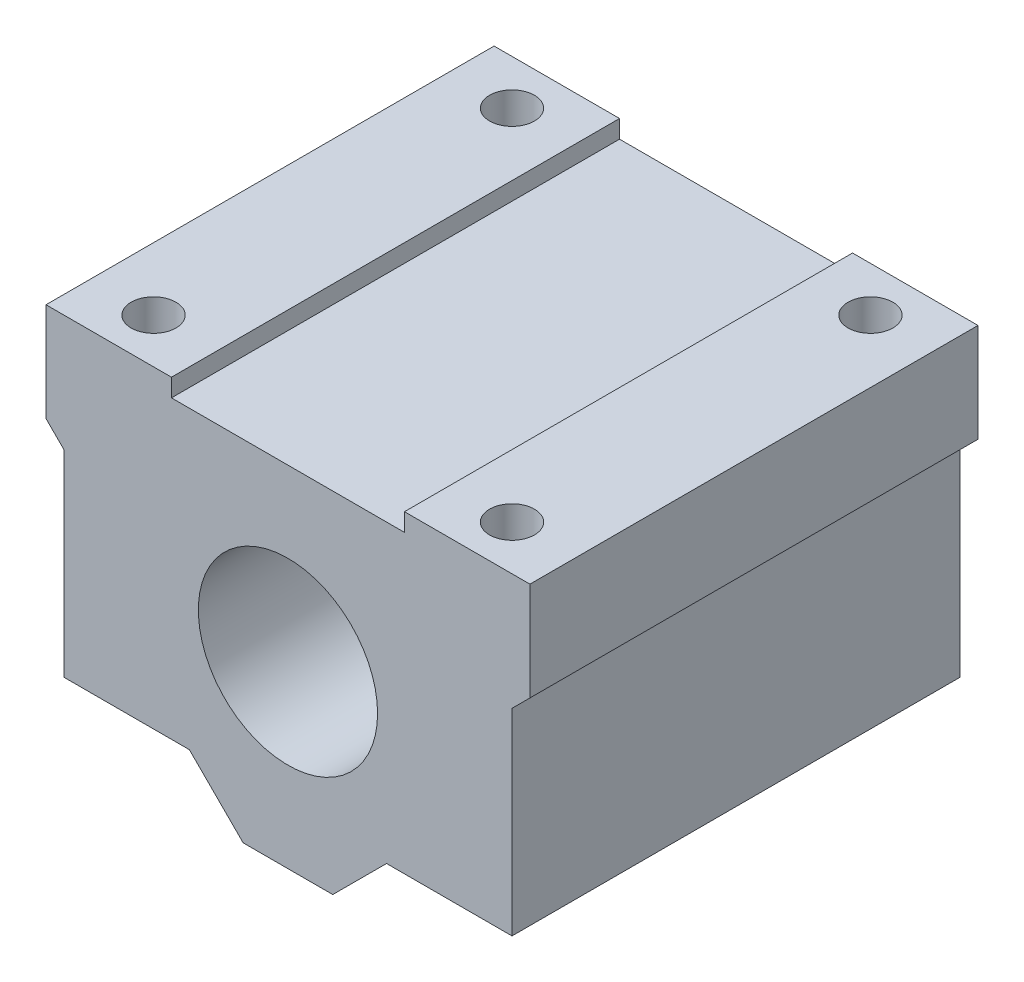
SolidWorks part; units mm, degrees
material "OTHER"
ref_plane "前视基准面" through (0, 0, 0) normal (0, 0, 1) x (1, 0, 0)
ref_plane "上视基准面" through (0, 0, 0) normal (0, 1, 0) x (1, 0, 0)
ref_plane "右视基准面" through (0, 0, 0) normal (1, 0, 0) x (0, 0, -1)
sketch "草图1" plane through (0, 0, 0) normal (0, 0, 1) x (1, 0, 0)
  line L0 (0, 43.497) -> (0, -42.9068) construction
  line L1 (5, -20) -> (-5, -20)
  line L2 (-5, -20) -> (-11, -14)
  line L3 (-11, -14) -> (-25, -14)
  line L4 (-25, -14) -> (-25, 8)
  line L5 (-25, 8) -> (-27, 10)
  line L6 (-27, 10) -> (-27, 21)
  line L7 (-27, 21) -> (-13, 21)
  line L8 (-13, 21) -> (-13, 19)
  line L9 (-13, 19) -> (13, 19)
  line L10 (13, 21) -> (13, 19)
  line L11 (27, 21) -> (13, 21)
  line L12 (27, 10) -> (27, 21)
  line L13 (25, 8) -> (27, 10)
  line L14 (25, -14) -> (25, 8)
  line L15 (11, -14) -> (25, -14)
  line L16 (5, -20) -> (11, -14)
  circle A0 centre (0, 0) radius 10
  point P16 (0, 19)
  point P23 (0, -20)
  dimension "D1" = 20
  dimension "D2" = 21
  dimension "D3" = 27
  dimension "D4" = 35
  dimension "D5" = 41
  dimension "D6" = 2
  dimension "D7" = 14
  dimension "D8" = 11
  dimension "D9" = 2
  dimension "D10" = 225
  dimension "D11" = 135
  dimension "D12" = 14
extrude "拉伸1" add sketch "草图1" along normal blind 50
hole_wizard "M6x1.0 螺纹孔1" positions "草图3" profile "草图2" tap size "M6x1.0" standard "ISO"
sketch "草图3" plane through (0, 21, 0) normal (0, 1, 0) x (-1, 0, 0)
  line L0 (-27, 50) -> (-27, 0) construction
  line L1 (-27, 0) -> (-13, 0) construction
  point P0 (-20, 5)
  dimension "D1" = 7
  dimension "D2" = 5
cosmetic thread "孔螺蚊线1" parameters "D1"=12, "D2"=6
sketch "草图2" plane through (20, 21, 5) normal (1, 0, 0) x (0, 0, 1)
  line L0 (0, 0) -> (0, 18.5022)
  line L1 (0, 18.5022) -> (2.5, 17)
  line L2 (2.5, 17) -> (2.5, 0)
  line L5 (2.5, 0) -> (0, 0)
  line L10 (0, 18.5022) -> (-2.5, 17) construction
  line L11 (0, -6.35) -> (0, 107.95) construction
  dimension "蹟恇謂郰芛眻噤" = 5
  dimension "蹟恇謂郰芛旮僅" = 17
  dimension "絳芛褒僅" = 118
pattern_linear "阵列(线性)1" count 2 spacing 40 along (0, 0, 1) count 2 spacing 40 along (-1, 0, 0) of "M6x1.0 螺纹孔1"
